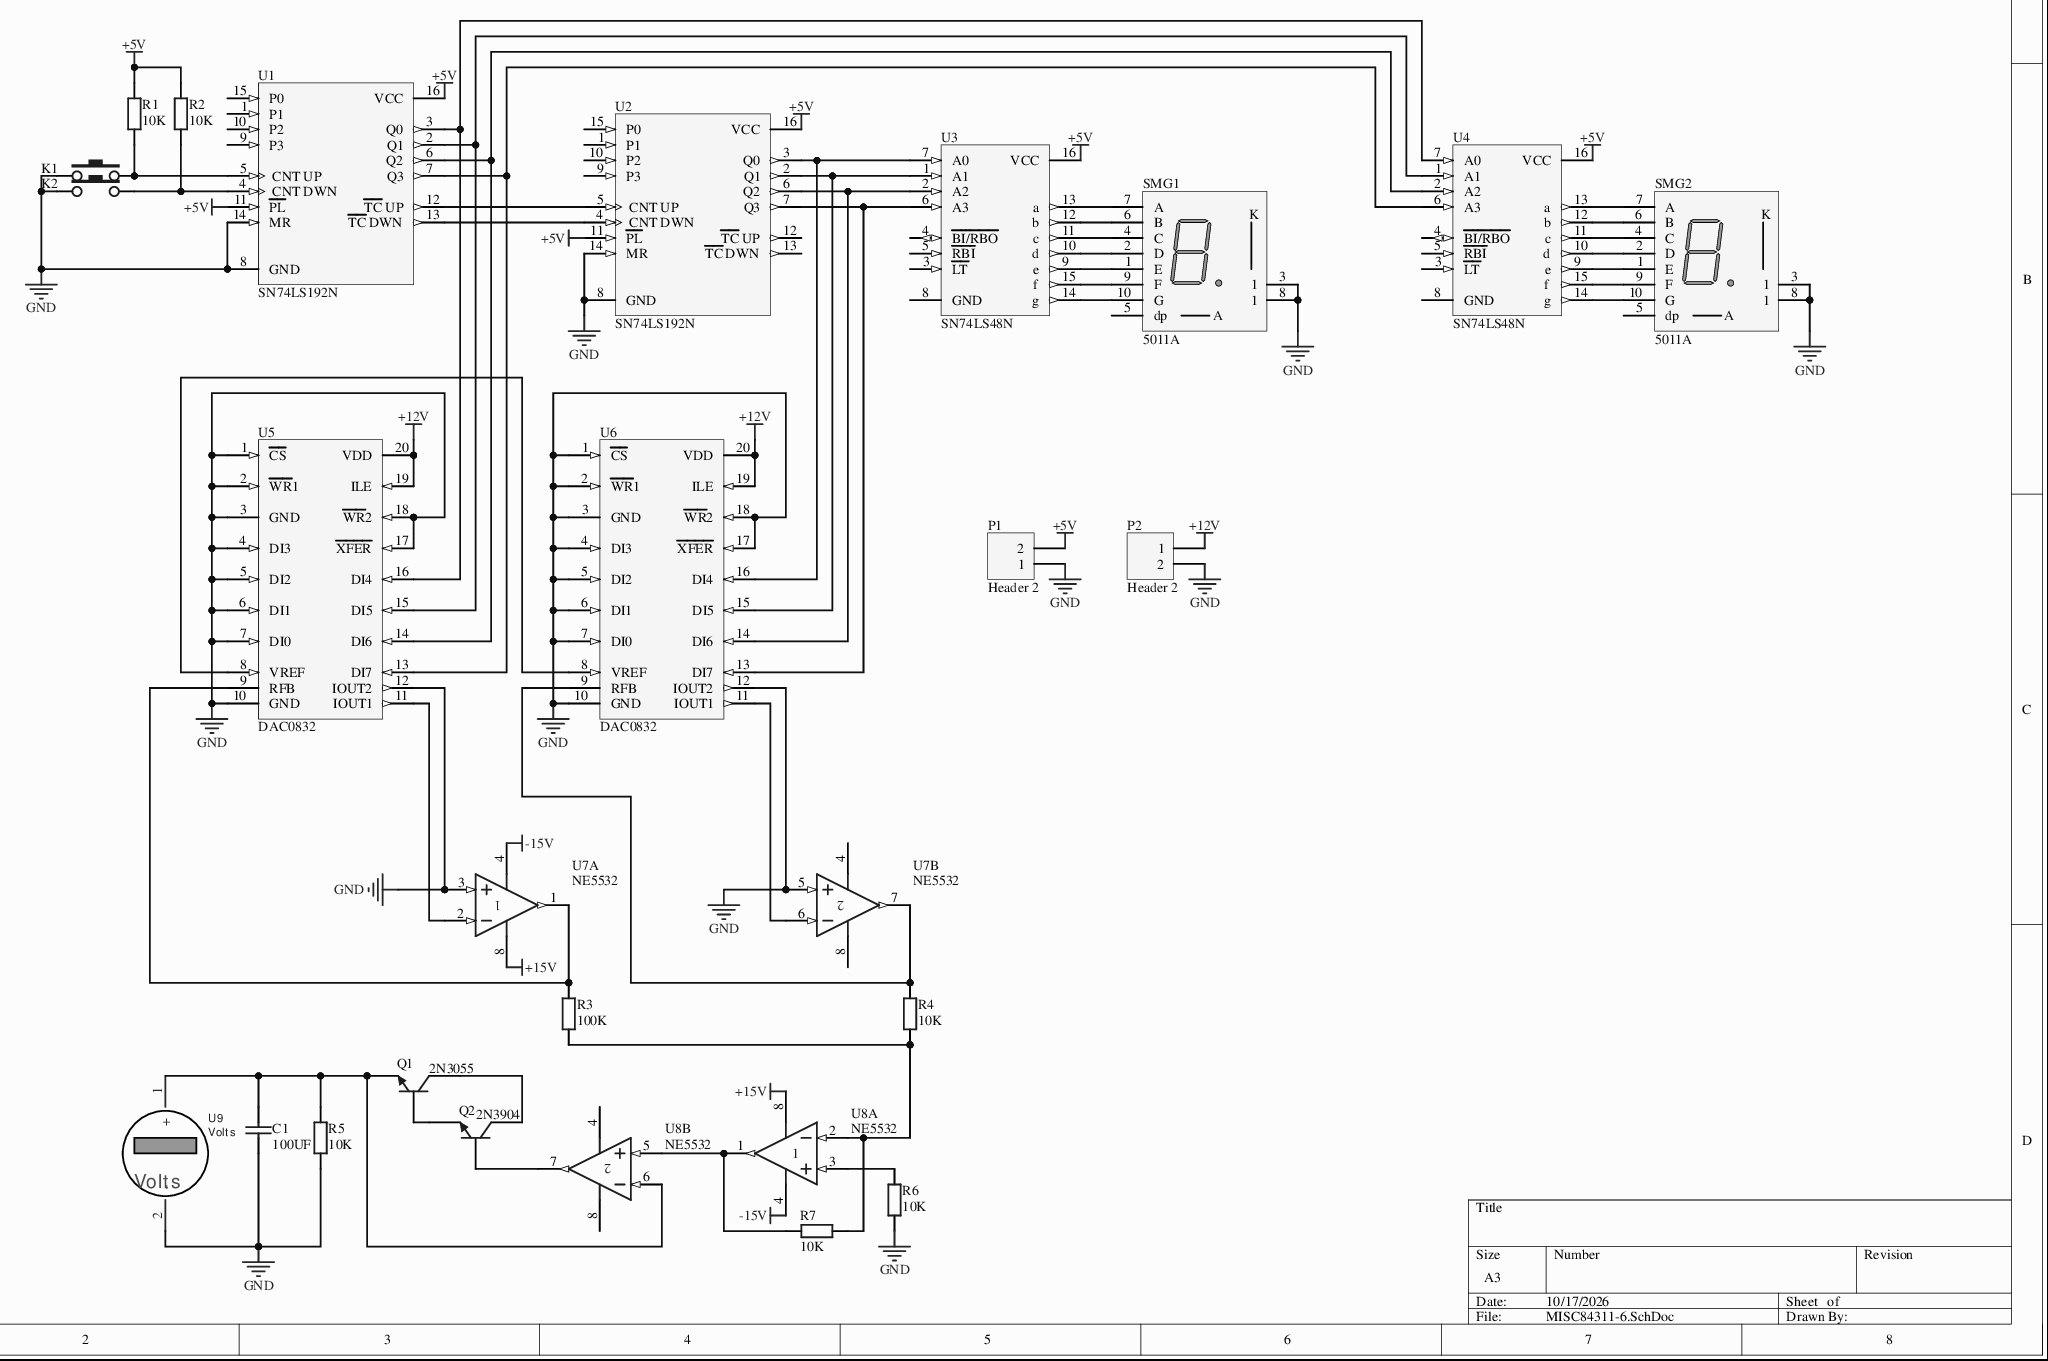
[diagram p0: MISC84311-6.SchDoc]
# Altium project MISC84311-2.PrjPcb
1 sheet, 25 parts. Net scope: global (net labels, ports and power ports of the same name join across sheets).
Board file: MISC84311.PcbDoc

## Sheet MISC84311-6.SchDoc
size A3

### Parts
C1  100UF  [RAD-0.3]
K1  KEY  [DIP-3X6X4.3]  (value not drawn)
K2  KEY  [DIP-3X6X4.3]  (value not drawn)
P1  Header 2  [HDR1X2]
P2  Header 2  [HDR1X2]
Q1  2N3055  [TO-92A]
Q2  2N3904  [TO-92A]
R1  10K  [RS 1/4W]
R2  10K  [RS 1/4W]
R3  100K  [RS 1/4W]
R4  10K  [RS 1/4W]
R5  10K  [RS 1/4W]
R6  10K  [RS 1/4W]
R7  10K  [RS 1/4W]
SMG1  5011A  [SMG 0.5-1P]
SMG2  5011A  [SMG 0.5-1P]
U1  SN74LS192N  [648-08]
U2  SN74LS192N  [648-08]
U3  SN74LS48N  [N016D]
U4  SN74LS48N  [N016D]
U5  DAC0832  [J20A]
U6  DAC0832  [J20A]
U7  NE5532  [P008]  (parts A,B of 2)
U8  NE5532  [P008]  (parts A,B of 2)
U9  Volts  [CAPACITANCE 1 FARAD 5,5 VOLT]

### Nets
+5V: P1.2 R1.2 R2.2 U1.11(~{PL}) U1.16(VCC) U2.11(~{PL}) U2.16(VCC) U3.16(VCC) U4.16(VCC)
+12V: P2.1 U5.19(ILE) U5.20(VDD) U6.19(ILE) U6.20(VDD)
+15V: U7.8(V+) U8.8(V+)
-15V: U7.4(V-) U8.4(V-)
GND: C1.1 K1.1 K2.1 P1.1 P2.2 R5.2 R6.1 SMG1.3(1) SMG1.8(1) SMG2.3(1) SMG2.8(1) U1.8(GND) U1.14(MR) U2.8(GND) U2.14(MR) U5.1(~{CS}) U5.2(~{WR}1) U5.3(GND) U5.4(DI3) U5.5(DI2) U5.6(DI1) U5.7(DI0) U5.10(GND) U5.12(IOUT2) U5.17(~{XFER}) U5.18(~{WR}2) U6.1(~{CS}) U6.2(~{WR}1) U6.3(GND) U6.4(DI3) U6.5(DI2) U6.6(DI1) U6.7(DI0) U6.10(GND) U6.12(IOUT2) U6.17(~{XFER}) U6.18(~{WR}2) U7.3(IN+) U7.5(IN+) U9.2(-)
NetC1_2: C1.2 Q1.1(E) R5.1 U8.6(IN-) U9.1(+)
NetK1_3: K1.3 R1.1 U1.5(CNT_UP)
NetK2_3: K2.3 R2.1 U1.4(CNT_DWN)
NetQ1_2: Q1.2(B) Q2.1(E)
NetQ1_3: Q1.3(C) Q2.3(C)
NetQ2_2: Q2.2(B) U8.7(OUT)
NetR3_1: R3.1 R4.1 R7.1 U8.2(IN-)
NetR3_2: R3.2 U5.9(RFB) U7.1(OUT)
NetR4_2: R4.2 U6.9(RFB) U7.7(OUT)
NetR6_2: R6.2 U8.3(IN+)
NetR7_2: R7.2 U8.1(OUT) U8.5(IN+)
NetSMG1_1: SMG1.1(E) U3.9(e)
NetSMG1_2: SMG1.2(D) U3.10(d)
NetSMG1_4: SMG1.4(C) U3.11(c)
NetSMG1_6: SMG1.6(B) U3.12(b)
NetSMG1_7: SMG1.7(A) U3.13(a)
NetSMG1_9: SMG1.9(F) U3.15(f)
NetSMG1_10: SMG1.10(G) U3.14(g)
NetSMG2_1: SMG2.1(E) U4.9(e)
NetSMG2_2: SMG2.2(D) U4.10(d)
NetSMG2_4: SMG2.4(C) U4.11(c)
NetSMG2_6: SMG2.6(B) U4.12(b)
NetSMG2_7: SMG2.7(A) U4.13(a)
NetSMG2_9: SMG2.9(F) U4.15(f)
NetSMG2_10: SMG2.10(G) U4.14(g)
NetU1_2: U1.2(Q1) U4.1(A1) U5.15(DI5)
NetU1_3: U1.3(Q0) U4.7(A0) U5.16(DI4)
NetU1_6: U1.6(Q2) U4.2(A2) U5.14(DI6)
NetU1_7: U1.7(Q3) U4.6(A3) U5.13(DI7)
NetU1_12: U1.12(~{TC}_UP) U2.5(CNT_UP)
NetU1_13: U1.13(~{TC}_DWN) U2.4(CNT_DWN)
NetU2_2: U2.2(Q1) U3.1(A1) U6.15(DI5)
NetU2_3: U2.3(Q0) U3.7(A0) U6.16(DI4)
NetU2_6: U2.6(Q2) U3.2(A2) U6.14(DI6)
NetU2_7: U2.7(Q3) U3.6(A3) U6.13(DI7)
NetU5_8: U5.8(VREF) U6.8(VREF)
NetU5_11: U5.11(IOUT1) U7.2(IN-)
NetU6_11: U6.11(IOUT1) U7.6(IN-)

Not connected (* = marked no-connect by the designer): SMG1 5(dp); SMG2 5(dp); U1 1(P1) 9(P3) 10(P2) 15(P0); U2 1(P1) 9(P3) 10(P2) 12(~{TC}_UP) 13(~{TC}_DWN) 15(P0); U3 3(~{LT}) 4(~{BI/RBO}) 5(~{RBI}) 8(GND); U4 3(~{LT}) 4(~{BI/RBO}) 5(~{RBI}) 8(GND)

### Library data of the parts
C1 = Cap: Capacitor; Value: 100pF; Published: 8-Jun-2000; LatestRevisionDate: 17-Jul-2002; LatestRevisionNote: Re-released for DXP Platform.; PackageReference: RAD-0.3; PackageDescription: Radial Cap, Thru-Hole; 2 Leads; 0.3 in Pin Spacing; Publisher: Altium Limited
P1 P2 = Header 2: Header, 2-Pin; LatestRevisionDate: 17-Jul-2002; LatestRevisionNote: Re-released for DXP Platform.; Publisher: Altium Limited
Q1 Q2 = 2N3904: NPN General Purpose Amplifier; Published: 8-Jun-2000; LatestRevisionDate: 15-Jan-2003; LatestRevisionNote: PCB Footprint 'BCY-W3/D4.7' replaced; DatasheetVersion: 1997; PackageVersion: Sep-1998; PackageReference: TO-92A; PackageDescription: TO, Flat Index; 3 In-Line, Axial Leads; Body Dia. 4.5mm; Leads 0.51 x 0.48 mm (max); ComponentLink1Description: Manufacturer Link; ComponentLink2Description: Datasheet; ComponentLink2URL: http://www.fairchildsemi.com/ds/2N%2F2N3904.pdf; Publisher: Altium Limited
R1-R7 = R-S: Color-band resistor; BOM名称: Color-band resistor
SMG1 SMG2 = 5011A: 0.5-inch 1-digit common-cathode seven-segment display; BOM名称: 0.5-inch 1-digit common-cathode
U1 U2 = SN74LS192N: Presettable BCD Decade Up/Down Counter; Package Information: Latest Revision: Apr-2000; Code - JEDEC: MS-001-BB; Published: 15-Apr-2002; Datasheet: Latest Revision: 18/10/1996; Package Reference: 648-08; Publisher: Altium Limited
U3 U4 = SN74LS48N: BCD-to-Seven-Segment Decoder/Driver; Revision 1: 12-Jul-2000: SIM Model Added.; Revision 2: 17-Jul-2002: Re-released for DXP Platform.; Package Information: Latest Revision: Oct-1995; Code - JEDEC: MS-001-BB; Published: 8-Jun-2000; Datasheet: 1988 TTL Logic Data Book (Mar-1988); Package Reference: N016D; Publisher: Altium Limited
U5 U6 = DAC0832LCJ: 8-Bit uP-Compatible, Double-Buffered Digital-to-Analog Converter; Package Information: Latest Revision: 2000; Code - JEDEC: MS-015-AE; Published: 15-Apr-2002; Datasheet: Latest Revision: May-1999; Package Reference: J20A; Publisher: Altium Limited
U7 U8 = NE5532AP: Dual Low-Noise Operational Amplifier; Package Information: Latest Revision: Jun-1999; Code - JEDEC: MO-001-AN; Published: 15-Apr-2002; Datasheet: Linear Circuits Data Book 1989 Volume 1 (May-1988); Package Reference: P008; Publisher: Altium Limited